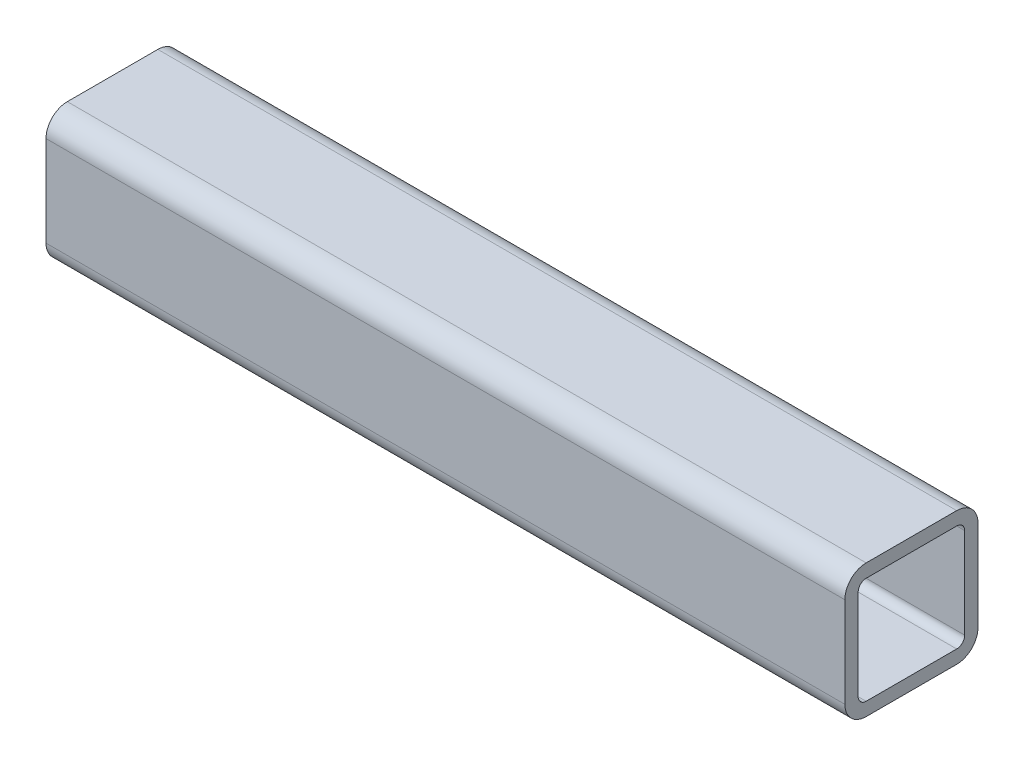
from build123d import *

# Parameters (mm, degrees)
COLD_FORMED_SQUARE_HOLLOW_SECTION_GB_T_6_DEPTH = 300


with BuildPart() as part:
    # Sketch1 → Cold-formed square hollow section GB/T 6728-2002 50 X 50 X 4(1) (new body)
    with BuildSketch(Plane.YZ.offset(-88.434077868)):
        with BuildLine():
            Line((-17, -25), (17, -25))
            ThreePointArc((17, -25), (22.656854249, -22.656854249), (25, -17))
            Line((25, -17), (25, 17))
            ThreePointArc((25, 17), (22.656854249, 22.656854249), (17, 25))
            Line((17, 25), (-17, 25))
            ThreePointArc((-17, 25), (-22.656854249, 22.656854249), (-25, 17))
            Line((-25, 17), (-25, -17))
            ThreePointArc((-25, -17), (-22.656854249, -22.656854249), (-17, -25))
        make_face()
        with BuildLine():
            Line((-17, -20), (17, -20))
            ThreePointArc((17, -20), (19.121320344, -19.121320344), (20, -17))
            Line((20, -17), (20, 17))
            ThreePointArc((20, 17), (19.121320344, 19.121320344), (17, 20))
            Line((17, 20), (-17, 20))
            ThreePointArc((-17, 20), (-19.121320344, 19.121320344), (-20, 17))
            Line((-20, 17), (-20, -17))
            ThreePointArc((-20, -17), (-19.121320344, -19.121320344), (-17, -20))
        make_face(mode=Mode.SUBTRACT)
    extrude(amount=COLD_FORMED_SQUARE_HOLLOW_SECTION_GB_T_6_DEPTH)


solid = part.part
